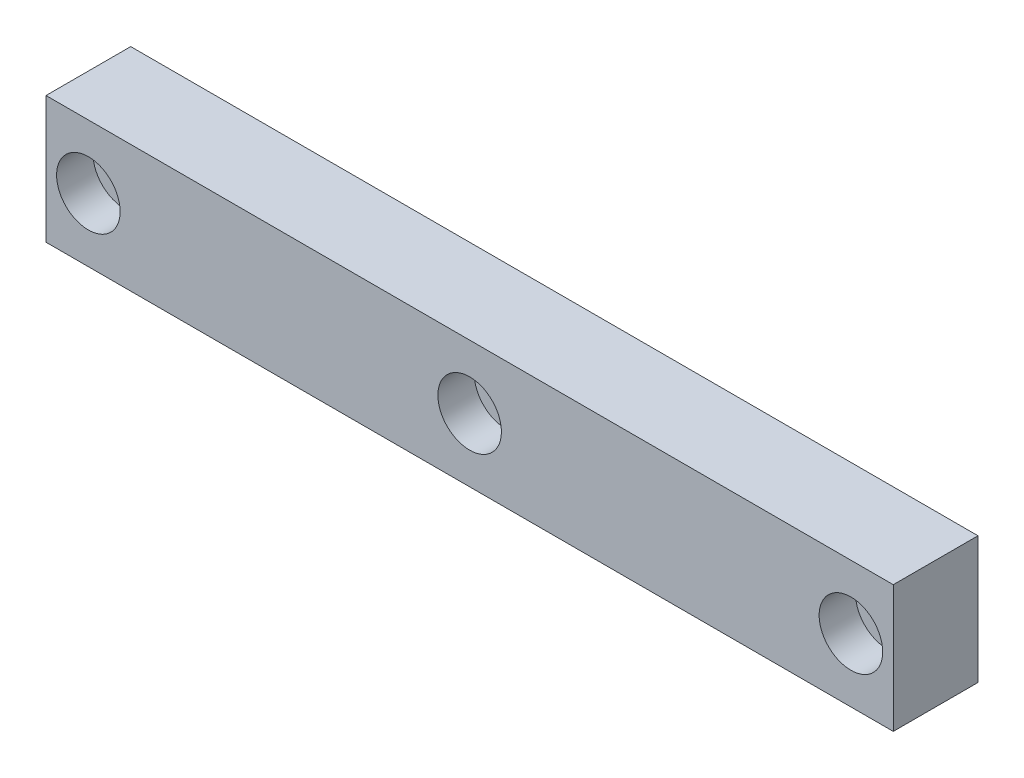
SolidWorks part; units mm, degrees
material "普通碳钢"
ref_plane "前视基准面" through (0, 0, 0) normal (0, 0, 1) x (1, 0, 0)
ref_plane "上视基准面" through (0, 0, 0) normal (0, 1, 0) x (1, 0, 0)
ref_plane "右视基准面" through (0, 0, 0) normal (1, 0, 0) x (0, 0, -1)
sketch "草图1" plane through (0, 0, 0) normal (0, 0, 1) x (1, 0, 0)
  line L1 (-100, -15) -> (100, -15)
  line L2 (-100, -15) -> (-100, 15)
  line L3 (-100, 15) -> (100, 15)
  line L4 (100, -15) -> (100, 15)
  line L5 (-100, -15) -> (100, 15) construction
  line L6 (-100, 15) -> (100, -15) construction
  point P0 (0, 0)
  dimension "D1" = 200
  dimension "D2" = 30
extrude "凸台-拉伸1" add sketch "草图1" along normal blind 20
hole_wizard "M8 六角凹头螺钉的柱形沉头孔1" positions "草图4" profile "草图2" counterbore size "M8" standard "Iso" end condition through all
sketch "草图4" plane through (0, 0, 20) normal (0, 0, 1) x (1, 0, 0)
  line L1 (-100, -15) -> (100, -15) construction
  point P0 (0, 0)
  point P3 (90, 0)
  point P5 (-90, 0)
  dimension "D1" = 90
  dimension "D2" = 90
  dimension "D3" = 15
  dimension "D4" = 15
sketch "草图2" plane through (0, 0, 20) normal (1, 0, 0) x (0, -1, 0)
  line L0 (0, 0) -> (0, 20)
  line L1 (0, 20) -> (4.5, 20)
  line L3 (4.5, 20) -> (4.5, 8.6)
  line L4 (4.5, 8.6) -> (7.5, 8.6)
  line L5 (7.5, 8.6) -> (7.5, 0)
  line L7 (7.5, 0) -> (0, 0)
  line L11 (0, -6.35) -> (0, 107.95) construction
  dimension "通孔孔直径" = 9
  dimension "通孔孔深度" = 20
  dimension "柱形沉头孔直径" = 15
  dimension "柱形沉头孔深度" = 8.6
